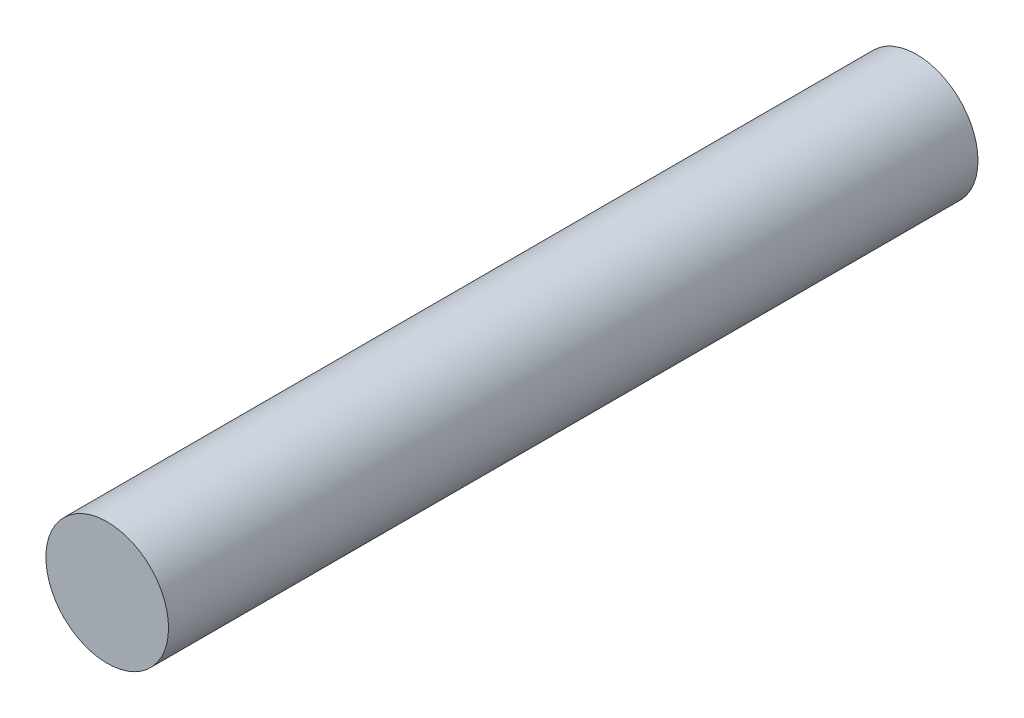
SolidWorks part; units mm, degrees
ref_plane "前视基准面" through (0, 0, 0) normal (0, 0, 1) x (1, 0, 0)
ref_plane "上视基准面" through (0, 0, 0) normal (0, 1, 0) x (1, 0, 0)
ref_plane "右视基准面" through (0, 0, 0) normal (1, 0, 0) x (0, 0, -1)
sketch "草图1" plane through (0, 0, 0) normal (0, 0, 1) x (1, 0, 0)
  circle A0 centre (0, 0) radius 12.5
  dimension "D1" = 25
extrude "凸台-拉伸1" add sketch "草图1" along normal blind 165
